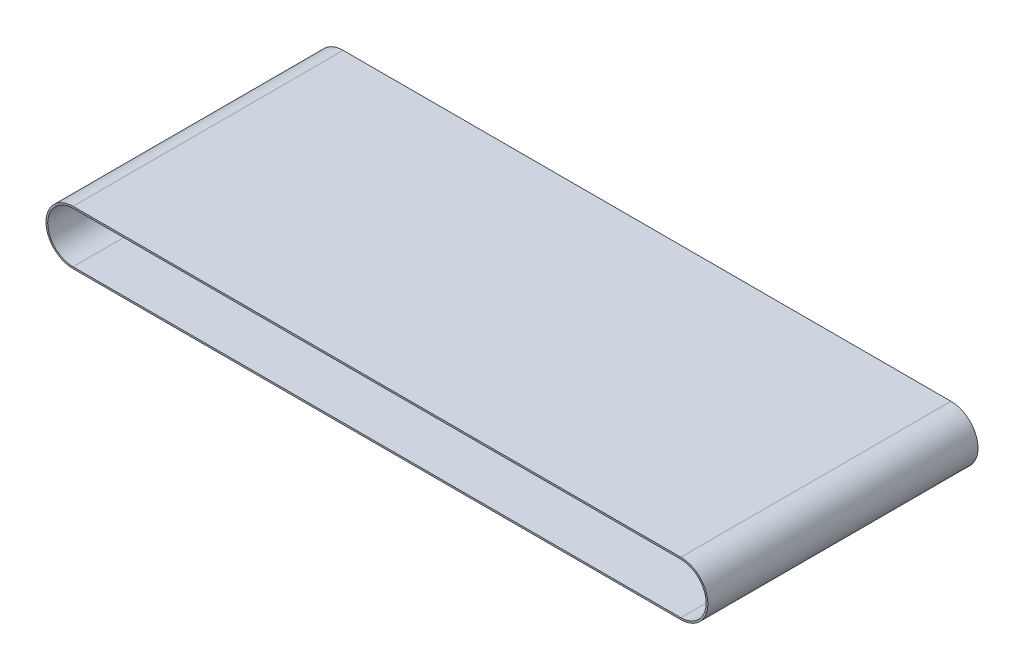
from build123d import *

# Parameters (mm, degrees)
EXTRUDE_1_DEPTH = 800


with BuildPart() as part:
    # 草图1 → 拉伸-薄壁1 (new body)
    with BuildSketch(Plane.XY):
        with BuildLine():
            Line((1800, -80), (0, -80))
            ThreePointArc((0, -80), (-80, 0), (0, 80))
            Line((0, 80), (1800, 80))
            ThreePointArc((1800, 80), (1880, 0), (1800, -80))
        make_face()
        with BuildLine():
            Line((1800, -75), (0, -75))
            ThreePointArc((0, -75), (-75, 0), (0, 75))
            Line((0, 75), (1800, 75))
            ThreePointArc((1800, 75), (1875, 0), (1800, -75))
        make_face(mode=Mode.SUBTRACT)
    extrude(amount=EXTRUDE_1_DEPTH)


solid = part.part
